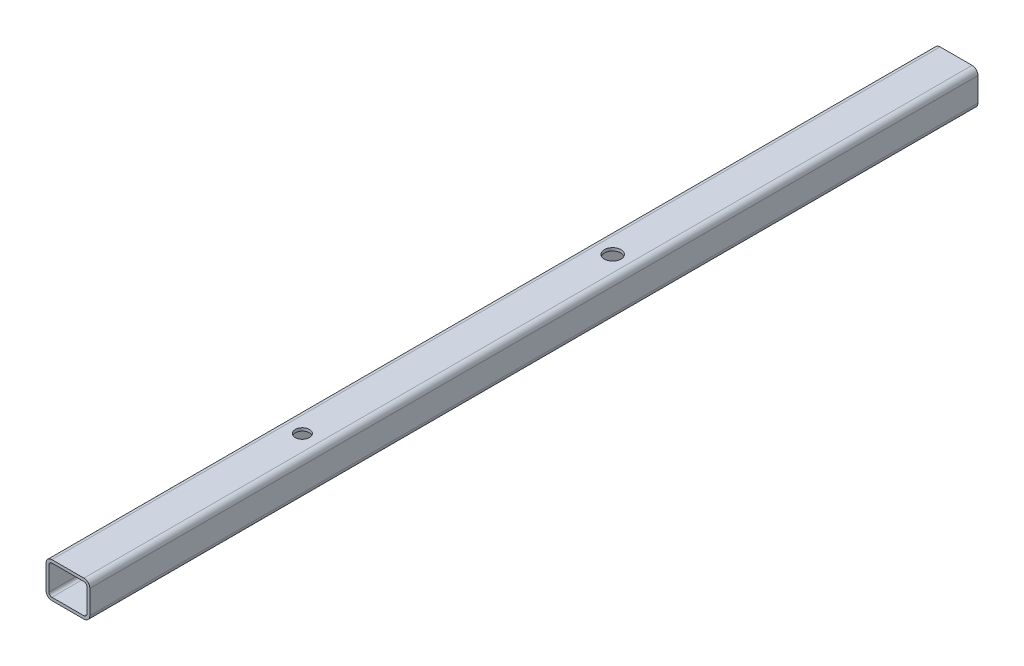
SolidWorks part; units mm, degrees
ref_plane "前视基准面" through (0, 0, 0) normal (0, 0, 1) x (1, 0, 0)
ref_plane "上视基准面" through (0, 0, 0) normal (0, 1, 0) x (1, 0, 0)
ref_plane "右视基准面" through (0, 0, 0) normal (1, 0, 0) x (0, 0, -1)
sketch "尺寸草图" plane through (0, 0, 0) normal (0, 0, 1) x (1, 0, 0)
  line L0 (-25.8313, 0) -> (16, 0) construction
  line L1 (0, 56.0755) -> (0, -63.3818) construction
  line L2 (-13.5, 12.5) -> (13.5, 12.5)
  line L3 (-13.5, 15) -> (13.5, 15)
  line L4 (-18.5, 10) -> (-18.5, -10)
  line L5 (-13.5, -15) -> (13.5, -15)
  line L6 (18.5, 10) -> (18.5, -10)
  line L7 (16, 10) -> (16, -10)
  line L8 (-13.5, -12.5) -> (13.5, -12.5)
  line L9 (-16, 10) -> (-16, -10)
  line L10 (-18.5, 15) -> (-18.5, -15) construction
  line L11 (-18.5, -15) -> (18.5, -15) construction
  line L12 (-16, -12.5) -> (16, -12.5) construction
  line L13 (-16, 12.5) -> (-16, -12.5) construction
  line L14 (16, 12.5) -> (16, -12.5) construction
  line L15 (18.5, 15) -> (18.5, -15) construction
  line L16 (-16, 12.5) -> (16, 12.5) construction
  line L17 (-18.5, 15) -> (18.5, 15) construction
  arc A0 (-18.5, -10) -> (-13.5, -15) centre (-13.5, -10) ccw
  arc A1 (-13.5, -12.5) -> (-16, -10) centre (-13.5, -10) cw
  arc A2 (16, -10) -> (13.5, -12.5) centre (13.5, -10) cw
  arc A3 (13.5, -15) -> (18.5, -10) centre (13.5, -10) ccw
  arc A4 (13.5, 12.5) -> (16, 10) centre (13.5, 10) cw
  arc A5 (13.5, 15) -> (18.5, 10) centre (13.5, 10) cw
  arc A6 (-13.5, 12.5) -> (-16, 10) centre (-13.5, 10) ccw
  arc A7 (-13.5, 15) -> (-18.5, 10) centre (-13.5, 10) ccw
  dimension "D2" = 5
  dimension "H" = 30
  dimension "B" = 37
  dimension "t" = 2.5
extrude "凸台-拉伸1" add sketch "尺寸草图" along normal blind 200 and the other way blind 300
sketch "草图7" plane through (0, 15, 0) normal (0, 1, 0) x (1, 0, 0)
  circle A0 centre (0, -2) radius 6
  dimension "D1" = 12
extrude "切除-拉伸2" cut sketch "草图7" against normal blind 83
sketch "草图8" plane through (0, 15, 0) normal (0, 1, 0) x (1, 0, 0)
  line L0 (13.5, 300) -> (-13.5, 300) construction
  circle A0 centre (0, 260) radius 7
  dimension "D2" = 14
  dimension "D1" = 40
extrude "切除-拉伸3" cut sketch "草图8" against normal through all both and the other way through all
sketch "草图11" plane through (0, 0, -300) normal (0, 0, -1) x (-1, 0, 0)
  line L0 (-13.5, 12.5) -> (13.5, 12.5) construction
  line L1 (-16, -12.5) -> (13.5, -12.5)
  line L2 (-16, -12.5) -> (-16, 10)
  line L3 (-13.5, 12.5) -> (13.5, 12.5)
  line L4 (18.5, -10) -> (18.5, 10)
  line L5 (13.5, 15) -> (-13.5, 15)
  line L6 (-18.5, 10) -> (-18.5, -10)
  line L7 (-13.5, -15) -> (13.5, -15)
  line L8 (18.5, -10) -> (18.5, 10)
  line L9 (13.5, 15) -> (-13.5, 15)
  line L10 (-18.5, 10) -> (-18.5, -10)
  line L11 (-13.5, -15) -> (13.5, -15)
  line L12 (16, -10) -> (16, 10)
  line L13 (-16, -12.5) -> (16, 12.5) construction
  line L14 (-16, 12.5) -> (16, -12.5) construction
  line L15 (16, 10) -> (16, -10) construction
  arc A0 (-16, 10) -> (-13.5, 12.5) centre (-13.5, 10) cw
  arc A1 (16, 10) -> (13.5, 12.5) centre (13.5, 10) ccw
  arc A2 (13.5, -12.5) -> (16, -10) centre (13.5, -10) ccw
  arc A4 (13.5, -15) -> (18.5, -10) centre (13.5, -10) ccw
  arc A5 (18.5, 10) -> (13.5, 15) centre (13.5, 10) ccw
  arc A6 (-13.5, 15) -> (-18.5, 10) centre (-13.5, 10) ccw
  arc A7 (-18.5, -10) -> (-13.5, -15) centre (-13.5, -10) ccw
  arc A8 (13.5, -15) -> (18.5, -10) centre (13.5, -10) ccw
  arc A9 (18.5, 10) -> (13.5, 15) centre (13.5, 10) ccw
  arc A10 (-13.5, 15) -> (-18.5, 10) centre (-13.5, 10) ccw
  arc A11 (-18.5, -10) -> (-13.5, -15) centre (-13.5, -10) ccw
  point P0 (0, 0)
  dimension "D2" = 2.5
  dimension "D1" = 0
extrude "凸台-拉伸4" add sketch "草图11" along normal blind 250
